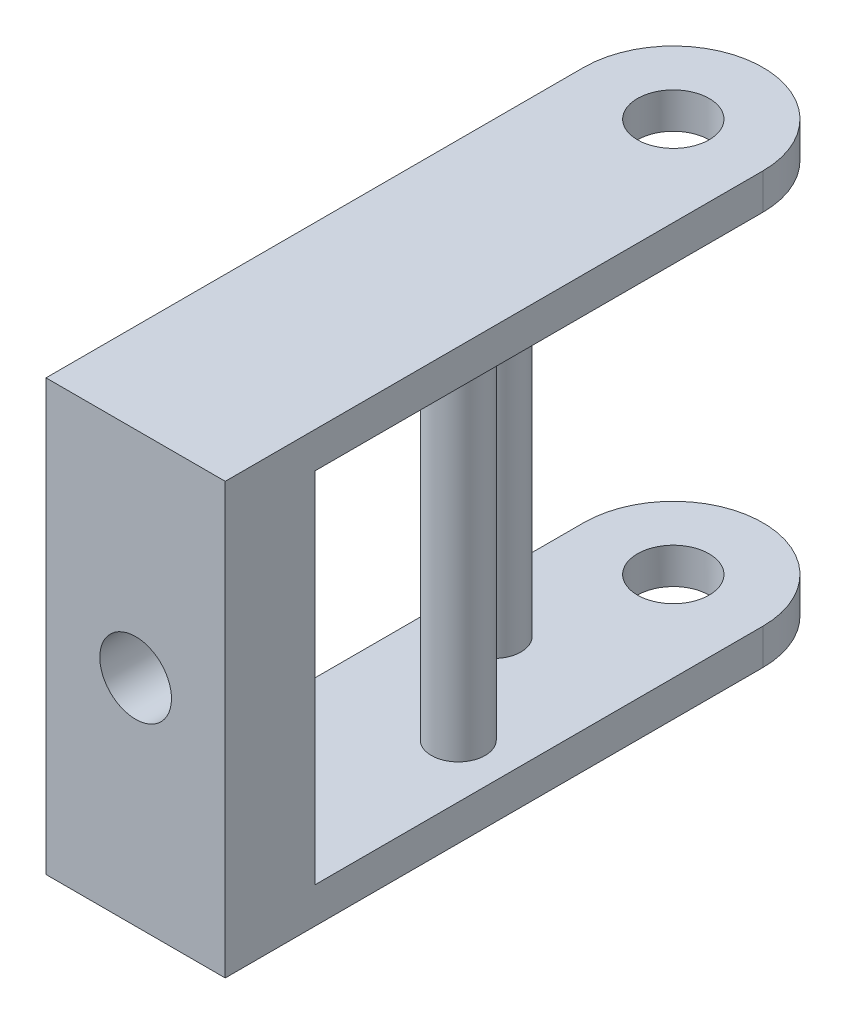
from build123d import *

# Parameters (mm, degrees)
BOSS_EXTRUDE1_DEPTH     = 24
CUT_EXTRUDE2_DEPTH      = 39.742741256
CUT_EXTRUDE2_DEPTH_BACK = 39.742741256
SKETCH4_R               = 2
CUT_EXTRUDE3_DEPTH      = 39.742741256
CUT_EXTRUDE3_DEPTH_BACK = 39.742741256
SKETCH6_W               = 32.588779774
SKETCH6_H               = 20
SKETCH7_R               = 2
CUT_EXTRUDE4_DEPTH      = 39.742741256
SKETCH8_R               = 1.5
BOSS_EXTRUDE3_DEPTH     = 22


with BuildPart() as part:
    # Sketch1 → Boss-Extrude1 (new body)
    with BuildSketch(Plane(origin=(0, 0, 0), x_dir=(1, 0, 0), z_dir=(0, 1, 0))):
        with BuildLine():
            Line((-5, 0), (-5, -30))
            Line((-5, -30), (5, -30))
            Line((5, -30), (5, 0))
            ThreePointArc((5, 0), (0, 5), (-5, 0))
        make_face()
    extrude(amount=BOSS_EXTRUDE1_DEPTH)

    # Sketch4 → Cut-Extrude2 (cut, two sides: drawn at the far end of the back side and taken through both)
    with BuildSketch(Plane(origin=(0, 24, 0), x_dir=(1, 0, 0), z_dir=(0, 1, 0)).offset(-CUT_EXTRUDE2_DEPTH_BACK)):
        with Locations(Location((0, 0, 0), (0, 0, 270))):
            Circle(SKETCH4_R)
    extrude(amount=CUT_EXTRUDE2_DEPTH + CUT_EXTRUDE2_DEPTH_BACK, mode=Mode.SUBTRACT)

    # Sketch6 → Cut-Extrude3 (cut, two sides: drawn at the far end of the back side and taken through both)
    with BuildSketch(Plane(origin=(0, 0, 0), x_dir=(0, 0, -1), z_dir=(1, 0, 0)).offset(-CUT_EXTRUDE3_DEPTH_BACK)):
        with Locations((-8.705610113, 12)):
            Rectangle(SKETCH6_W, SKETCH6_H)
    extrude(amount=CUT_EXTRUDE3_DEPTH + CUT_EXTRUDE3_DEPTH_BACK, mode=Mode.SUBTRACT)

    # Sketch7 → Cut-Extrude4 (cut, through all)
    with BuildSketch(Plane(origin=(0, 0, 25), x_dir=(-1, 0, 0), z_dir=(0, 0, -1))):
        with Locations(Location((0, 12, 0), (0, 0, 90))):
            Circle(SKETCH7_R)
    extrude(amount=-CUT_EXTRUDE4_DEPTH, mode=Mode.SUBTRACT)

    # Sketch8 → Boss-Extrude3 (add)
    with BuildSketch(Plane(origin=(0, 24, 0), x_dir=(1, 0, 0), z_dir=(0, 1, 0))):
        with Locations(Location((-2, -8, 0), (0, 0, 270))):
            Circle(SKETCH8_R)
        with Locations(Location((2, -14, 0), (0, 0, 270))):
            Circle(SKETCH8_R)
    extrude(amount=-BOSS_EXTRUDE3_DEPTH)


solid = part.part
